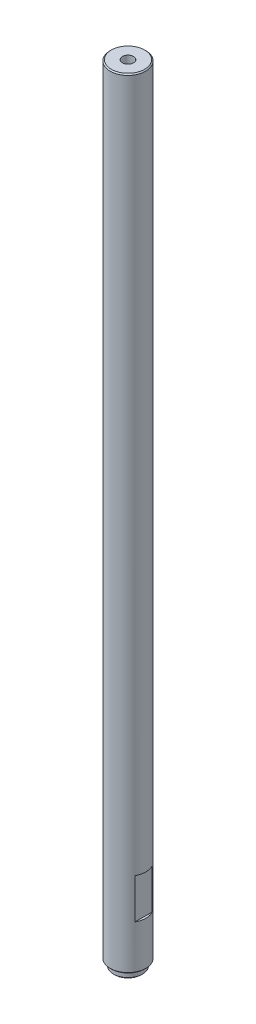
SolidWorks part; units mm, degrees
material "SUJ2"
ref_plane "Front Plane" through (0, 0, 0) normal (0, 0, 1) x (1, 0, 0)
ref_plane "Top Plane" through (0, 0, 0) normal (0, 1, 0) x (1, 0, 0)
ref_plane "Right Plane" through (0, 0, 0) normal (1, 0, 0) x (0, 0, -1)
sketch "Sketch1" plane through (0, 0, 0) normal (0, 1, 0) x (1, 0, 0)
  circle A0 centre (0, 0) radius 8
  dimension "D1" = 16
extrude "Boss-Extrude1" add sketch "Sketch1" along normal mid plane 350
hole_wizard "M6 Tapped Hole1" positions "Sketch6" profile "Sketch7" tap size "M6" standard "GB"
sketch "Sketch6" plane through (0, 175, 0) normal (0, 1, 0) x (1, 0, 0)
  point P0 (0, 0)
sketch "Sketch7" plane through (0, 175, 0) normal (1, 0, 0) x (0, 0, 1)
  line L0 (0, 0) -> (0, 16.5022)
  line L1 (0, 16.5022) -> (2.5, 15)
  line L2 (2.5, 15) -> (2.5, 0)
  line L5 (2.5, 0) -> (0, 0)
  line L10 (0, 16.5022) -> (-2.5, 15) construction
  line L11 (0, -6.35) -> (0, 107.95) construction
  dimension "螺纹孔钻头直径" = 5
  dimension "螺纹孔钻头深度" = 15
  dimension "导头角度" = 118
cosmetic thread "Hole thread 1" parameters "D1"=12, "D2"=6
mirror "Mirror1" about plane through (0, 0, 0) normal (0, 1, 0) of "M6 Tapped Hole1"
sketch "Sketch8" plane through (0, -175, 0) normal (0, -1, 0) x (1, 0, 0)
  line L1 (-7, 15.0953) -> (7, 15.0953)
  line L2 (-7, 15.0953) -> (-7, -15.0953)
  line L3 (-7, -15.0953) -> (7, -15.0953)
  line L4 (7, 15.0953) -> (7, -15.0953)
  line L5 (-7, 15.0953) -> (7, -15.0953) construction
  line L6 (-7, -15.0953) -> (7, 15.0953) construction
  point P0 (0, 0)
  dimension "D1" = 14
extrude "Cut-Extrude1" cut sketch "Sketch8" against normal blind 18 from offset 20 flip side to cut offset against normal yes
sketch "Sketch9" plane through (0, -175, 0) normal (0, -1, 0) x (1, 0, 0)
  circle A0 centre (0, 0) radius 6.5
  dimension "D1" = 13
extrude "Boss-Extrude2" add sketch "Sketch9" along normal blind 3
hole_wizard "M6 Tapped Hole2" positions "Sketch10" profile "Sketch11" tap size "M6" standard "ISO"
sketch "Sketch10" plane through (0, -178, 0) normal (0, -1, 0) x (-1, 0, 0)
  point P0 (0, 0)
sketch "Sketch11" plane through (0, -178, 0) normal (1, 0, 0) x (0, 0, -1)
  line L0 (0, 0) -> (0, 18.5022)
  line L1 (0, 18.5022) -> (2.5, 17)
  line L2 (2.5, 17) -> (2.5, 0)
  line L5 (2.5, 0) -> (0, 0)
  line L10 (0, 18.5022) -> (-2.5, 17) construction
  line L11 (0, -6.35) -> (0, 107.95) construction
  dimension "螺纹孔钻头直径" = 5
  dimension "螺纹孔钻头深度" = 17
  dimension "导头角度" = 118
cosmetic thread "Hole thread 2" parameters "D1"=12, "D2"=6
chamfer "Chamfer1" distance 0.5 angle 45 2 edges at (0, -175, 8) (0, -178, -6.5)
chamfer "Chamfer2" distance 0.5 angle 45 1 edges at (0, 175, 8)
